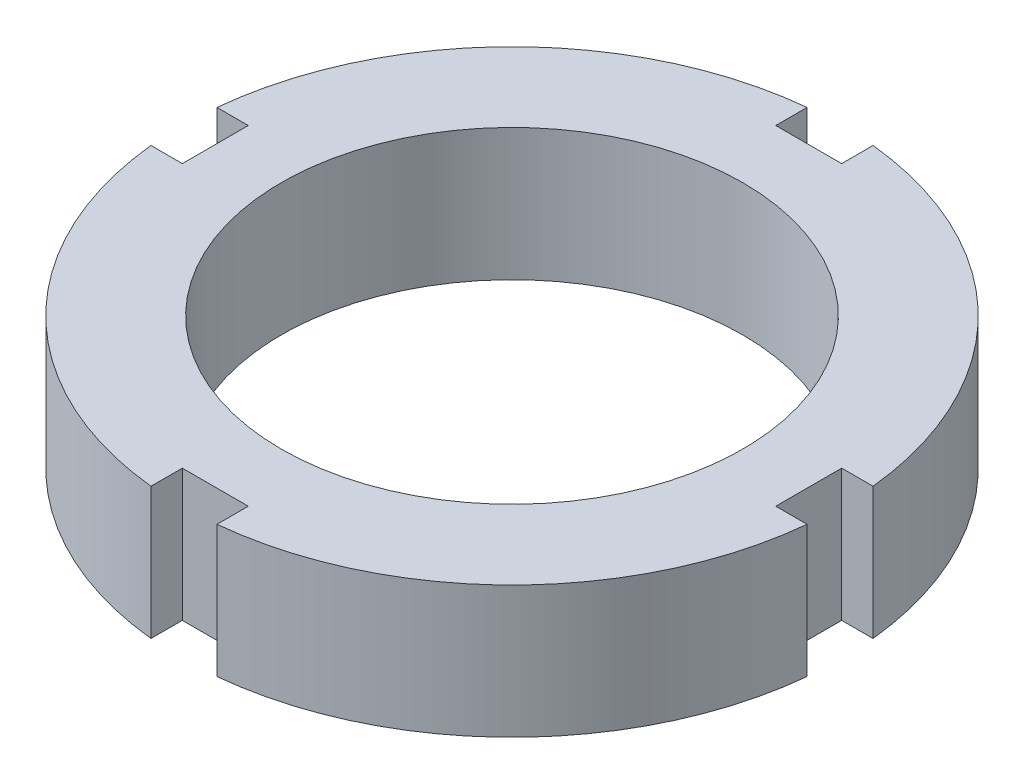
from build123d import *

# Parameters (mm, degrees)
SKETCH1_R           = 35
BOSS_EXTRUDE1_DEPTH = 20


with BuildPart() as part:
    # Sketch1 → Boss-Extrude1 (new body)
    with BuildSketch(Plane(origin=(0, 0, 0), x_dir=(1, 0, 0), z_dir=(0, 1, 0))):
        with BuildLine():
            Line((-5, 49.749371855), (-5, 45))
            Line((-5, 45), (5, 45))
            Line((5, 45), (5, 49.749371855))
            ThreePointArc((5, 49.749371855), (35.355339059, 35.355339059), (49.749371855, 5))
            Line((49.749371855, 5), (45, 5))
            Line((45, 5), (45, -5))
            Line((45, -5), (49.749371855, -5))
            ThreePointArc((49.749371855, -5), (35.355339059, -35.355339059), (5, -49.749371855))
            Line((5, -49.749371855), (5, -45))
            Line((5, -45), (-5, -45))
            Line((-5, -45), (-5, -49.749371855))
            ThreePointArc((-5, -49.749371855), (-35.355339059, -35.355339059), (-49.749371855, -5))
            Line((-49.749371855, -5), (-45, -5))
            Line((-45, -5), (-45, 5))
            Line((-45, 5), (-49.749371855, 5))
            ThreePointArc((-49.749371855, 5), (-35.355339059, 35.355339059), (-5, 49.749371855))
        make_face()
        with Locations(Location((0, 0, 0), (0, 0, 270))):
            Circle(SKETCH1_R, mode=Mode.SUBTRACT)
    extrude(amount=BOSS_EXTRUDE1_DEPTH)


solid = part.part
